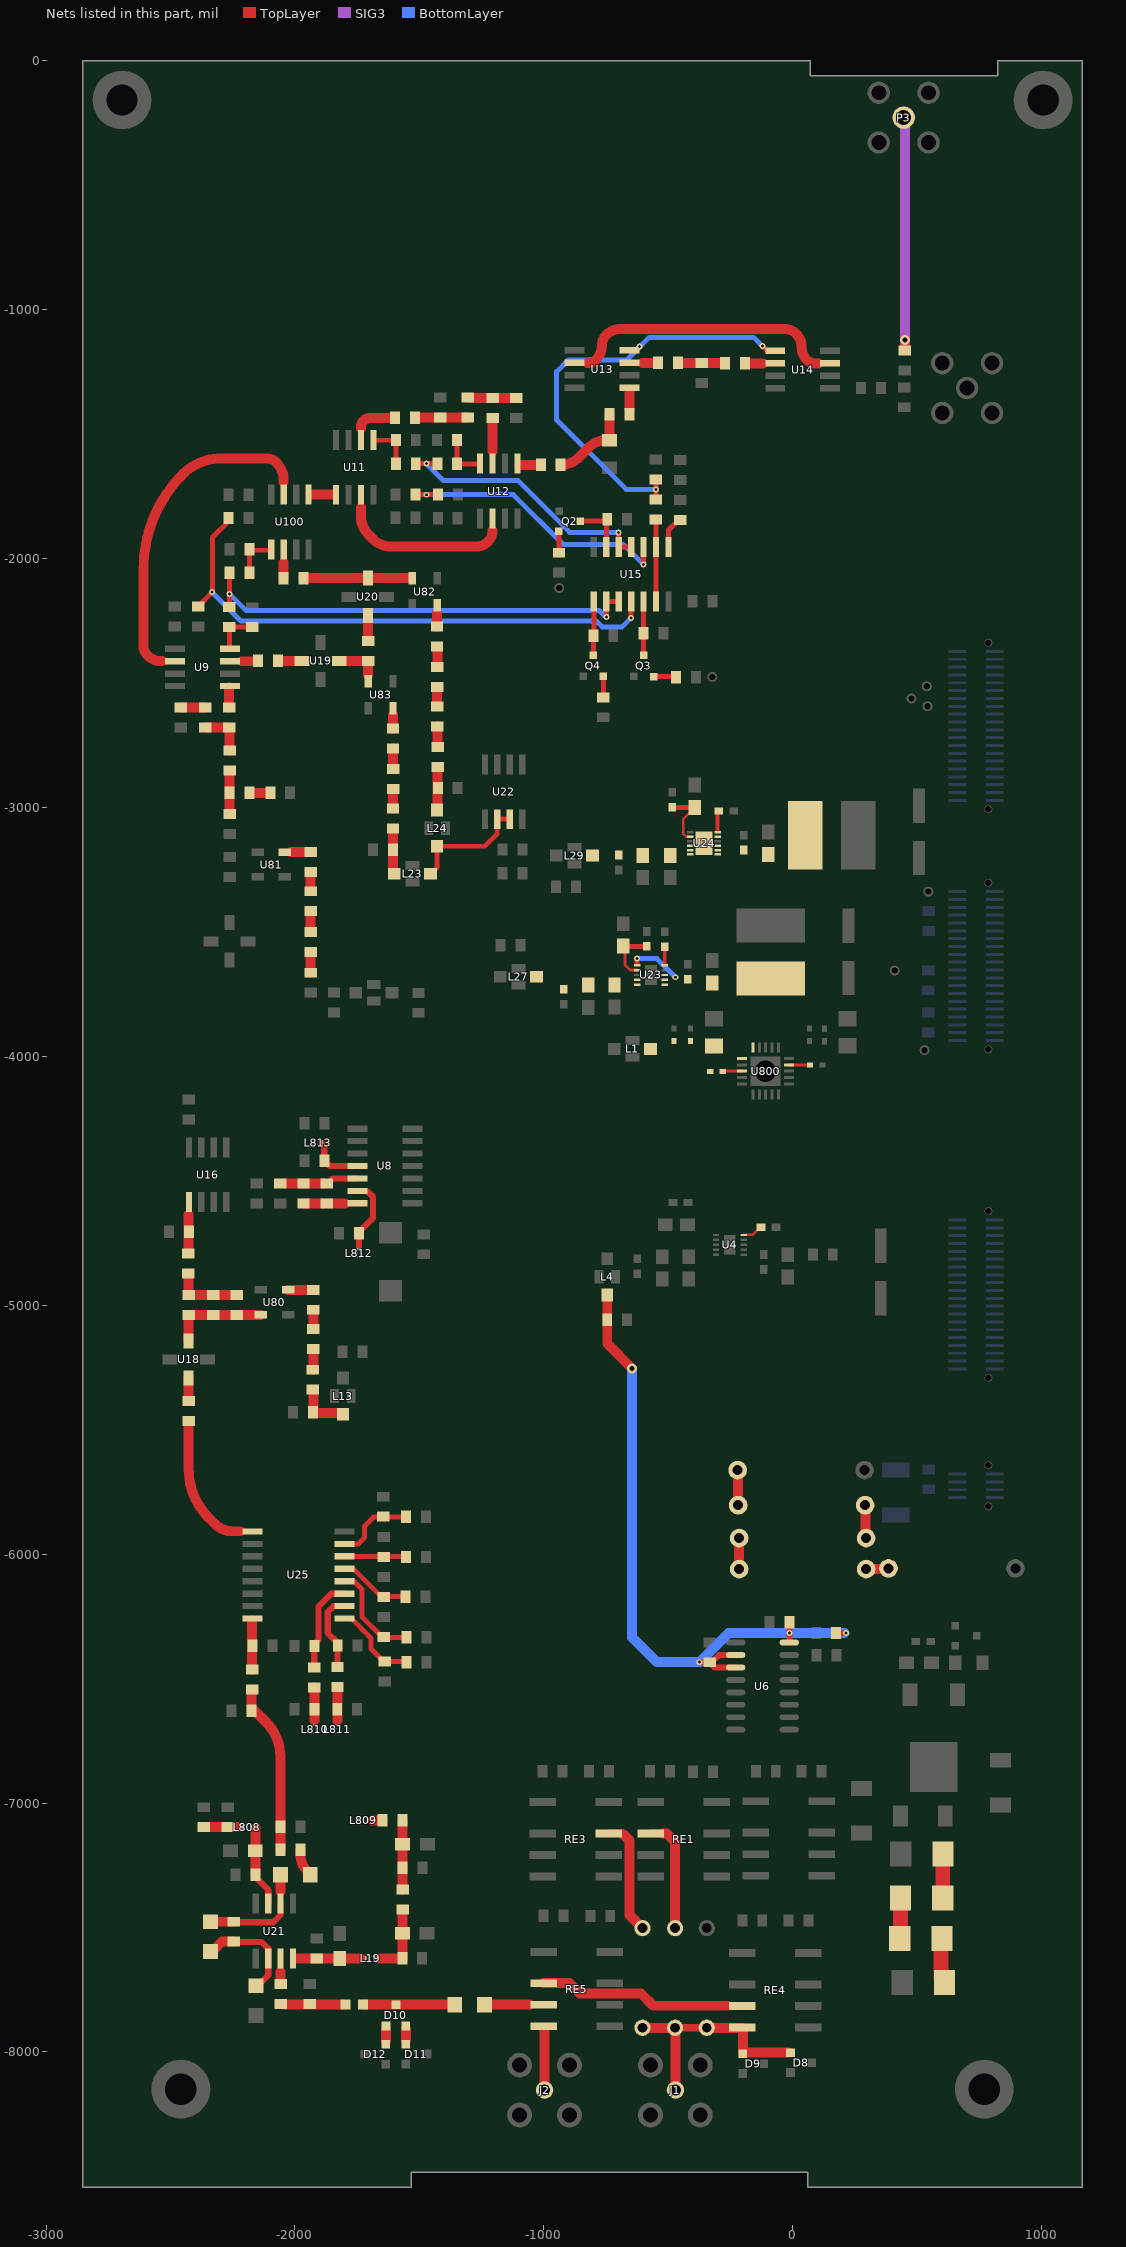
[diagram p0: the nets of this part, all layers, seen from the top]
# Altium PCB MISC109560.PcbDoc (part 6 of 7)
Units mil, origin at the board's own origin, x right, y up, seen from the top; angles counter-clockwise.
Board outline 4015.75 x 8543.31 mil, 4 copper layers (TopLayer, GND, SIG3, BottomLayer); 280 components, 173 nets, 936 pads, 3695 vias.

## Via types
v1: diameter 24, hole 12, TopLayer to BottomLayer, 3659 vias
v2: diameter 20, hole 12, TopLayer to BottomLayer, 32 vias
v3: diameter 40, hole 20, TopLayer to BottomLayer, 4 vias

## Nets (pads, with @x,y where several pads share a name; then routed paths per layer and width w, separated by ;. In a path a pad name is that pad's centre, name@x,y a point inside that pad or via, vN(x,y) a via of type N, cw(c..) or ccw(c..) an arc to the next point about the centre after c; other vN are vias at no path point) (continued)
NetC53_1: C53.1 C54.1 L15.1 | length 318.4
  TopLayer w40: C53.1@-932,-1623 -930.42,-1623 ccw(c-930.42,-1523) -859.71,-1593.71 -819.29,-1553.29 cw(c-748.58,-1624) -748.58,-1524 L15.1@-737,-1524 ; L15.1@-736,-1511 C54.1@-736,-1420
NetC53_2: C53.2 U12.1 | length 71
  TopLayer w40: U12.1@-1097,-1623 C53.2@-1026,-1623
NetC54_2: C54.2 U13.1 | length 72.6
  TopLayer w40: C54.2@-656,-1396.31 U13.1@-656,-1323.68
NetC55_1: C55.1 U13.3 | length 62.4
  TopLayer w40: -603.41,-1213.09 C55.1@-540.96,-1213.09
NetC55_2: C55.2 C56.1 L16.2 | length 182.1
  TopLayer w40: C55.2@-455.63,-1214.68 L16.2@-370,-1214.68 ; L16.2@-372,-1214.68 C56.1@-275.55,-1214.68
NetC56_2: C56.2 U14.6 | length 66.4
  TopLayer w40: C56.2@-185.96,-1216.09 -119.59,-1216.09
NetC57_1: C57.1 R41.1 U13.4 U14.5 | length 1839.7
  TopLayer w20: U13.4@-655.96,-1163.09 -629.41,-1163.09 -614,-1147.68 v1(-615,-1147.68) ; R41.1@-550,-1763.31 v1(-550,-1721.31) C57.1@-550,-1689.31 ; v1(-122,-1145.68) -102.59,-1165.09 U14.5@-69.96,-1165.09
  BottomLayer w20: -643,-1721.31 -603,-1721.31 ; v1@-608.5,-1142.18 -607,-1140.68 v1@-606,-1140.68 ; v1@-608,-1142.68 v1@-609,-1143.68 ; v1@-550,-1722.31 v1@-551,-1721.31 ; v1(-550,-1721.31) v1@-551,-1721.31 ; v1@-123,-1143.68 -126,-1140.68 v1@-127,-1140.68 ; v1(-122,-1145.68) v1@-127,-1140.68 ; v1@-609,-1143.68 -667,-1201.68 -901,-1201.68 -948,-1248.68 -948,-1442.68 -669.37,-1721.31 -603,-1721.31 ; v1@-609,-1143.68 v1@-606,-1140.68 ; v1@-606,-1140.68 -576,-1110.68 -157,-1110.68 v1@-127,-1140.68 ; -603,-1721.31 v1@-551,-1721.31
NetC58_1: C58.1 C65.1 | length 72
  TopLayer w40: C58.1@-2182,-2941.31 C65.1@-2110,-2941.31
NetC58_2: C58.2 L10.1 L11.1 | length 164.4
  TopLayer w40: L10.1@-2261.96,-3026.72 L11.1@-2261.96,-2862.31
NetC59_1: C59.1 L11.2 L12.1 | length 181.7
  TopLayer w40: C59.1@-2352,-2678.31 -2265,-2678.31 -2261.96,-2681.35 L11.2@-2261.96,-2771.72
NetC59_2: C59.2 C66.2 | length 98.6
  TopLayer w40: C66.2@-2459.59,-2597.72 C66.2@-2458.96,-2597.72 C59.2@-2360.96,-2597.72
NetC60_1: C60.1 R42.1 U9.4 | length 166.3
  TopLayer w20: U9.4@-2263.59,-2354.9 R42.1@-2263.59,-2274.27 C60.1@-2177.96,-2274.27
NetC61_2: C61.2 R43.2 U100.5 | length 173
  TopLayer w20: R43.2@-2183,-2056.31 -2183,-1966.31 U100.5@-2100,-1966.31
NetC62_2: C62.2 R44.1 U11.5 | length 171.3
  TopLayer w20: U11.5@-1672,-1524.31 -1595,-1524.31 -1594.41,-1524.9 R44.1@-1594.41,-1618.35
NetC63_2: C63.2 R45.1 U12.4 | length 181.1
  TopLayer w20: C63.2@-1348.41,-1523.35 -1348.41,-1614.72 -1342.82,-1620.31 U12.4@-1261,-1620.31
NetC64_2: C64.2 L13.3 R46.2 | length 191.2
  TopLayer w40: R46.2@-1927,-5347.26 -1926,-5348.26 C64.2@-1926,-5435 ; C64.2@-1926,-5433 L13.3@-1823,-5433
NetC67_1: C67.1 U18.1 | length 81.6
  TopLayer w40: C67.1@-2426.92,-5374.27 U18.1@-2426.92,-5292.72
NetC67_2: C67.2 U25.1 | length 555.4
  TopLayer w40: C67.2@-2426.96,-5465.31 -2426.96,-5658.26 ccw(c-2149.86,-5658.26) -2345.8,-5854.2 -2321.29,-5878.71 ccw(c-2250.58,-5808) -2250.58,-5908 -2219,-5908
NetC68_1: C68.1 C69.2 R49.2 R50.2 | length 269
  TopLayer w40: C69.2@-2426.96,-4881.31 C68.1@-2426.96,-4959.31 R49.2@-2235.96,-4959.31
NetC68_2: C68.2 R49.1 R50.1 U18.3 U80.1 | length 389.7
  TopLayer w40: U18.3@-2426.92,-5142.72 -2426.92,-5043.35 -2421.88,-5038.31 R50.1@-2328.96,-5038.31 R49.1@-2233.96,-5038.31 ; R49.1@-2232.26,-5038.31 U80.1@-2136.96,-5038.31
NetC69_1: C69.1 R53.2 U16.1 | length 152
  TopLayer w40: C69.1@-2426.96,-4787.31 -2426.96,-4635.31
NetC70_2: C70.2 C74.2 L18.1 L19.1 | length 273.5
  TopLayer w40: -1663,-7624 C74.2@-1574.48,-7624 ; C74.2@-1568.48,-7624 C70.2@-1568.48,-7523 L18.1@-1568.48,-7439
NetC71_2: C71.2 C75.2 L19.3 U21.4 | length 264
  TopLayer w40: U21.4@-1997.48,-7624 C75.2@-1912.48,-7624 C71.2@-1820.48,-7624 -1733.48,-7624
NetC72_1: C72.1 C73.2 L17.2 L18.2 | length 270
  TopLayer w40: L18.2@-1567.48,-7348 C72.1@-1567.48,-7260 C73.2@-1567.48,-7166 L17.2@-1567.48,-7078
NetC76_1: C76.1 U9.3 | length 54
  TopLayer w40: -2212,-2412.31 C76.1@-2158,-2412.31
NetC76_2: C76.2 U19.1 | length 84
  TopLayer w40: C76.2@-2065,-2411.31 U19.1@-1981,-2411.31
NetC77_1: C77.1 U19.3 U83.1 | length 165.7
  TopLayer w40: U19.3@-1822,-2411.31 C77.1@-1713,-2411.31 ; U83.1@-1706,-2468 C77.1@-1706,-2411.31
NetC77_2: C77.2 U20.1 | length 94
  TopLayer w40: C77.2@-1707,-2322.31 U20.1@-1707,-2228.31
NetC78_1: C78.1 U20.3 U82.1 | length 424.3
  TopLayer w40: C78.1@-1965,-2078.31 U20.3@-1707,-2078.31 U82.1@-1540.69,-2078.31
NetC78_2: C78.2 U100.6 | length 60.4
  TopLayer w40: C78.2@-2045,-2077.76 -2045,-2017.31
NetC79_1: C79.1 D10.3 R40.2 | length 369.5
  TopLayer w40: C79.1@-1727,-7810 R40.2@-1357.48,-7810
NetC79_2: C79.2 R58.2 R59.2 | length 237.1
  TopLayer w40: R58.2@-2044.07,-7809.41 C79.2@-1807,-7809.41
NetC80_2: C80.2 L20.2 L21.2 | length 204.4
  TopLayer w40: L20.2@-1513,-1433.31 L21.2@-1308.59,-1433.31
NetC81_2: C81.2 L21.1 L22.1 | length 184
  TopLayer w40: L21.1@-1295,-1354.31 C81.2@-1111,-1354.31
NetC82_1: C82.1 R60.2 | length 103.4
  TopLayer w40: C82.1@-1978.48,-7188 -1978.48,-7204.1 ccw(c-1878.48,-7204.1) -1949.19,-7274.81 R60.2@-1943,-7281
NetC82_2: C82.2 C116.1 R74.2 R82.2 | length 666.6
  TopLayer w40: R82.2@-2173.71,-6631 -2173.71,-6562.72 cw(c-2164.22,-6562.72) C116.1@-2170.93,-6556.01 ; R82.2@-2164,-6627 -2115.23,-6675.77 cw(c-2252.25,-6812.78) -2058.48,-6812.78 R74.2@-2058.48,-7095 ; C82.2@-2058.26,-7187.69 R74.2@-2058.26,-7100.22
NetC83_1: C83.1 C86.1 L808.1 U21.7 | length 407.3
  TopLayer w10: -2174,-7129 -2174,-7093 -2144,-7093 -2144,-7129
  TopLayer w25: C83.1@-2157.48,-7299 -2107.44,-7349.04 U21.7@-2107.44,-7404.41
  TopLayer w40: C86.1@-2159.26,-7191.41 -2159.26,-7108 ; C83.1@-2158.26,-7284.78 C86.1@-2158.26,-7189
NetC84_1: C84.1 L23.3 R62.2 | length 149.3
  TopLayer w40: L23.3@-1606,-3249 C84.1@-1606,-3174 ; C84.1@-1606,-3169.31 R62.2@-1606,-3095
NetC85_2: C85.2 L24.3 R65.1 | length 159.4
  TopLayer w40: L24.3@-1427,-3004.98 R65.1@-1427,-2845.61
NetC87_1: C87.1 R60.1 R69.1 U21.6 | length 418.7
  TopLayer w25: C87.1@-2263.48,-7479 -2122.48,-7479 -2087.48,-7479 -2057.48,-7449 -2057.48,-7426 U21.6@-2057.44,-7404.41
  TopLayer w40: R69.1@-2339.48,-7477 C87.1@-2251.48,-7477 ; -2058.09,-7355.39 R60.1@-2058.09,-7287.69
NetC87_2: C87.2 R61.2 R69.2 U21.2 | length 380
  TopLayer w25: C87.2@-2240.48,-7558 -2134.48,-7558 -2107.44,-7585.04 U21.2@-2107.44,-7624.41 -2107.44,-7691.96 R61.2@-2135.48,-7720
  TopLayer w40: R69.2@-2326,-7590 -2293,-7557 C87.2@-2250.48,-7557
NetC89_1: C89.1 L813.1 U8.11 | length 251.4
  TopLayer w10: L813.1@-1889.52,-4342 -1875,-4342 ; -1881.96,-4349 -1875,-4342.48 -1875,-4357
  TopLayer w25: C89.1@-1882,-4424.04 -1882,-4354 ; C89.1@-1882,-4419 C89.1@-1881.96,-4419.04 ; C89.1@-1881.96,-4419.31 C89.1@-1881.96,-4419.04 ; U8.11@-1748.37,-4440.35 -1860.65,-4440.35 C89.1@-1881.96,-4419.04
NetC90_1: C90.1 L32.2 L811.1 | length 134
  TopLayer w40: -1828.93,-6668 L32.2@-1828.93,-6534.01
NetC93_2: C93.2 C98.1 C99.2 L27.1 U23.9 U23.10
NetC94_2: C94.2 C95.1 L26.1 U23.1 U23.2 U23.3 U23.6 | length 205
  TopLayer w20: -625.14,-3627 v1(-625.14,-3607.14)
  BottomLayer w20: v1(-625.14,-3607.14) -545.86,-3607.14 v1(-471,-3682)
NetC96_1: C96.1 R70.1 U25.15 | length 298.6
  TopLayer w20: U25.15@-1792,-5959 -1746,-5959 -1720,-5933 -1720,-5887 -1683.69,-5850.69 R70.1@-1565.24,-5850.69
NetC101_1: C101.1 R72.1 U23.7 | length 203.2
  TopLayer w10: C101.1@-692,-3575 C101.1@-685,-3575
  TopLayer w12: C101.1@-674,-3580 -674,-3633 -653.75,-3653.25 U23.7@-625.14,-3653.25
  TopLayer w20: C101.1@-672,-3558 R72.1@-586,-3558
NetC102_1: C102.1 R73.1 U25.14 | length 244.4
  TopLayer w20: U25.14@-1800.71,-6008.69 R73.1@-1556.31,-6008.69
NetC104_1: C104.1 L812.1 U8.13 | length 294.8
  TopLayer w25: U8.13@-1748.37,-4540.35 -1710.65,-4540.35 -1686,-4565 -1686,-4648 -1742,-4704 -1742,-4764
NetC105_2: C105.2 L31.1 L810.1 | length 133
  TopLayer w40: -1921.93,-6669 L31.1@-1921.93,-6536.01
NetC109_1: C109.1 R75.1 U25.13 | length 276.1
  TopLayer w20: U25.13@-1800.71,-6058.69 U25.13@-1796,-6058.69 ; U25.13@-1796,-6057 -1767,-6057 -1695,-6129 C109.1@-1655,-6169 ; C109.1@-1657.93,-6171.01 R75.1@-1573.93,-6171.01
NetC110_2: C110.2 C113.1 C114.2 L29.1 U24.10 U24.11 U24.12
NetC111_2: C111.2 C112.1 L28.1 U24.1 U24.2 U24.3 U24.5 U24.13
NetC116_2: C116.2 R83.2 U25.8 | length 197.3
  TopLayer w40: U25.8@-2171.93,-6271.01 cw(c-2172.46,-6271.54) -2171.71,-6271.54 ; C116.2@-2171.71,-6463.69 U25.8@-2171.71,-6267.01
NetC118_1: C118.1 R77.1 U25.12 | length 399.3
  TopLayer w20: U25.12@-1800.71,-6108.69 U25.12@-1792,-6108.69 ; U25.12@-1792,-6108 -1763,-6108 -1731,-6140 -1731,-6251 -1648,-6334 R77.1@-1560,-6334
NetC119_1: C119.1 R81.1 U24.8 | length 243.4
  TopLayer w10: -435.5,-3109.53 -429.06,-3115.98 ; -435.5,-3109.5 -440,-3105 -440,-3047 C119.1@-393,-3000 ; -429.02,-3115.98 -427.26,-3117.74 U24.8@-411.41,-3117.74
  TopLayer w20: R81.1@-478,-3000 C119.1@-393,-3000
NetC128_2: C128.2 L31.2 U25.11 | length 370.5
  TopLayer w25: L31.2@-1921.93,-6448.01 C128.2@-1921.93,-6369.01 -1921.93,-6361.01 -1904.93,-6344.01 -1904.93,-6210.01 -1853.61,-6158.69 U25.11@-1800.71,-6158.69
NetC129_2: C129.2 L32.1 U25.10 | length 385.6
  TopLayer w20: -1865.93,-6276.01 -1865.93,-6231.01 -1843.61,-6208.69 U25.10@-1800.71,-6208.69 ; L32.1@-1828.93,-6448.01 L32.1@-1828.93,-6439.01
  TopLayer w25: -1843.61,-6208.69 -1844.61,-6208.69 -1867.93,-6232.01 -1867.93,-6317.01 -1828.93,-6356.01 L32.1@-1828.93,-6439.01
NetC130_1: C130.1 R84.1 U25.9 | length 337.5
  TopLayer w20: U25.9@-1800.71,-6258.69 U25.9@-1772,-6258.69 ; U25.9@-1772,-6260 -1732,-6300 -1724,-6308 -1695,-6337 -1695,-6379 C130.1@-1647,-6427 ; C130.1@-1649.93,-6432.01 R84.1@-1559.93,-6432.01
NetC803_1: C803.1 U800.14 | length 77.1
  TopLayer w12: U800.14@-14.02,-4033.9 C803.1@63.1,-4033.9
NetC804_1: C804.1 C805.1 C806.1 L1.1 R800.1 U800.1 U800.20
NetC809_1: C809.1 L25.2 L808.3 | length 137
  TopLayer w40: L25.2@-2366,-7097 C809.1@-2269,-7097 -2229,-7097
NetD2_1: D2.1 D3.2 | length 145
  TopLayer w60: D2.1@596,-7702 D3.2@596,-7557
NetD3_1: D3.1 D4.2 | length 146.5
  TopLayer w60: D3.1@433,-7527.54 D4.2@433,-7381
NetD4_1: D4.1 D5.2 | length 146
  TopLayer w60: D4.1@603,-7381 D5.2@603,-7235
NetD8_1: D8.1 D9.1 J1.5 R17.1 R20.1 R23.1 RE4.4 | length 938.4
  TopLayer w30: R23.1@-603.26,-7903 R23.1@-594.59,-7903 ; R17.1@-472.26,-7903 R20.1@-345.26,-7903 ; RE4.4@-201,-7908.59 RE4.4@-201,-7903.87
  TopLayer w40: R23.1@-595,-7902.59 -594.59,-7903 -594.38,-7903.21 R17.1@-472.26,-7903.21 ; R17.1@-472.26,-7903 R17.1@-472.26,-7903.21 ; J1.5@-471.26,-8153.31 -471.26,-7904.21 R17.1@-472.26,-7903.21 ; R20.1@-345.26,-7903.21 RE4.4@-201.66,-7903.21 ; RE4.4@-198,-7908.59 -199.5,-7910.09 -199.5,-8003.09 D8.1@-13.96,-8003.09
NetD10_1: D10.1 D12.2 | length 49.8
  TopLayer w40: D12.2@-1634.26,-7956.78 D10.1@-1634.26,-7907
NetD10_2: D10.2 D11.1 | length 47.8
  TopLayer w40: D11.1@-1554.26,-7952.78 D10.2@-1554.26,-7905
NetJ2_5: J2.5 RE5.4 | length 247.3
  TopLayer w40: J2.5@-997,-8153.31 RE5.4@-997,-7906
NetL12_2: L12.2 U9.1 | length 79.4
  TopLayer w40: L12.2@-2263.96,-2597.72 U9.1@-2263.96,-2518.35
NetL17_1: L17.1 L809.3 | length 42.5
  TopLayer w40: -1690,-7070 L17.1@-1647.48,-7070
NetL20_1: L20.1 U11.6 | length 163.5
  TopLayer w40: -1735,-1477.31 -1735,-1471.86 cw(c-1697.44,-1471.86) -1724,-1445.31 cw(c-1697.54,-1471.77) -1697.54,-1434.35 L20.1@-1598.41,-1434.35
NetL22_2: L22.2 U12.3 | length 133.6
  TopLayer w40: -1205.41,-1567.9 L22.2@-1205.41,-1434.35
NetL23_1: L23.1 L24.1 U22.6 U22.7 | length 472.8
  TopLayer w20: L23.1@-1440,-3253 -1429,-3242 L24.1@-1429,-3155.61 -1236.61,-3155.61 -1187,-3106 U22.6@-1187,-3042 ; U22.6@-1181,-3047 U22.7@-1136.69,-3047
NetP3_5: P3.5 R1.2 | length 922
  TopLayer w40: R1.2@452,-1154 v3(452,-1122)
  SIG3 w40: v3@452,-1121 P3.5@452,-231
NetQ2_2: Q2.2 R51.1 | length 80
  TopLayer w20: R51.1@-939,-1976.31 Q2.2@-939,-1896.31
NetQ2_3: Q2.3 R54.2 U15.13 | length 199.4
  TopLayer w20: Q2.3@-846,-1849.31 R54.2@-750,-1849.31 ; U15.13@-748.96,-1952.72 R54.2@-748.96,-1849.35
NetQ3_2: Q3.2 R52.1 | length 81
  TopLayer w20: Q3.2@-558,-2474.31 R52.1@-477,-2474.31
NetQ3_3: Q3.3 R55.1 U15.5 | length 207.6
  TopLayer w20: Q3.3@-598.96,-2380.31 U15.5@-598.96,-2172.72
NetQ4_2: Q4.2 R56.2 | length 80
  TopLayer w20: R56.2@-761,-2557.31 Q4.2@-761,-2477.31
NetQ4_3: Q4.3 R57.2 U15.1 | length 187.6
  TopLayer w20: Q4.3@-801,-2378.31 R57.2@-801,-2309.31 ; R57.2@-798.96,-2291.27 -798.96,-2173.31 U15.1@-798.96,-2172.72
NetR7_1: R7.1 R8.1 | length 132
  TopLayer w40: R8.1@-219,-5803.31 R7.1@-219,-5671.31
NetR8_2: R8.2 R9.2 | length 112
  TopLayer w40: R9.2@292,-5928.31 R8.2@292,-5816.31
NetR9_1: R9.1 R10.1 | length 105.4
  TopLayer w40: R10.1@-214.78,-6059.94 R9.1@-214.78,-5954.53
NetR10_2: R10.2 R11.2 | length 78
  TopLayer w40: R10.2@295,-6058.94 326,-6058.94 369.63,-6058.94 R11.2@372,-6061.31
NetR13_1: R13.1 U4.5 | length 68.8
  TopLayer w10: U4.5@-197,-4717.57 -161.57,-4717.57 R13.1@-138,-4694
NetR17_2: R17.2 RE1.2 | length 458
  TopLayer w30: RE1.2@-569.66,-7121.98 RE1.2@-522,-7121.98
  TopLayer w40: RE1.2@-522,-7122.59 -506,-7122.59 -472.26,-7156.33 R17.2@-472.26,-7503
NetR23_2: R23.2 RE3.7 | length 471.1
  TopLayer w30: RE3.7@-739.31,-7121.98 -680.61,-7121.98
  TopLayer w40: -683,-7123.59 -655,-7151.59 -655,-7451.26 R23.2@-603.26,-7503
NetR27_2: R27.2 R28.1 U15.4 | length 2218.9
  TopLayer w20: R27.2@-2388.59,-2192.27 v1@-2332,-2135.68 ; v1(-2333,-2134.68) v1@-2332,-2135.68 ; R28.1@-2264,-1847.31 -2332,-1915.31 v1@-2332,-2135.68 ; v1(-648.96,-2238.35) U15.4@-648.96,-2172.72
  BottomLayer w20: v1(-2333,-2134.68) -2217.37,-2250.31 -789.69,-2250.31 -765.69,-2274.31 -685,-2274.31 v1@-650,-2239.31
NetR29_2: R29.2 R30.2 U15.10 | length 1144.6
  TopLayer w20: R29.2@-1508.96,-1742.35 v1@-1472,-1742.35 ; v1(-1472,-1743.31) v1@-1472,-1742.35 ; R30.2@-1425.41,-1742.35 v1@-1472,-1742.35 ; v1(-598.96,-2024.27) U15.10@-598.96,-1952.72
  BottomLayer w20: v1@-1471,-1743 -1122.31,-1743 -923,-1942.31 -680.92,-1942.31 v1(-598.96,-2024.27)
NetR31_2: R31.2 U15.8 | length 121.1
  TopLayer w20: U15.8@-498.96,-1952.72 -498.96,-1885.27 R31.2@-461,-1847.31
NetR33_1: R33.1 R34.1 U8.14 | length 139.4
  TopLayer w40: R33.1@-1965.41,-4590.31 R34.1@-1887.96,-4590.31 ; R34.1@-1860.92,-4590.35 -1798.96,-4590.35
NetR33_2: R33.2 R34.2 R35.2 U8.12 | length 278
  TopLayer w25: R34.2@-1864.96,-4508.31 -1847,-4490.35 U8.12@-1748.37,-4490.35
  TopLayer w40: R35.2@-2038.96,-4510.31 R34.2@-1884.96,-4510.31
NetR36_2: R36.2 R37.1 | length 74.4
  TopLayer w40: R36.2@-1937.27,-3664 R37.1@-1937.27,-3589.63
NetR37_2: R37.2 R38.2 | length 59
  TopLayer w40: R37.2@-1937.27,-3493 R38.2@-1937.27,-3434.04
NetR38_1: R38.1 R39.1 | length 66.1
  TopLayer w40: R38.1@-1937.27,-3336.41 R39.1@-1937.27,-3270.27
NetR39_2: R39.2 U81.3 | length 78
  TopLayer w40: -2015,-3179 R39.2@-1937,-3179
NetR40_1: R40.1 RE5.3 | length 182
  TopLayer w40: R40.1@-1238,-7810 -1056,-7810
NetR41_2: R41.2 U15.6 U15.9 | length 317.4
  TopLayer w20: U15.6@-548.96,-2172.72 U15.9@-548.96,-1952.72 R41.2@-548.96,-1855.35
NetR42_2: R42.2 R43.1 U15.2 U15.3 | length 1787.9
  TopLayer w20: R42.2@-2263.59,-2194.27 v1(-2263.59,-2141.72) R43.1@-2263.59,-2068.72 ; v1(-748.96,-2235.35) U15.2@-748.96,-2172.72 ; U15.2@-747.41,-2172.72 U15.3@-698.96,-2172.72
  BottomLayer w20: v1(-2263.59,-2141.72) -2196,-2209.31 -776.69,-2209.31 v1@-751,-2235
NetR44_2: R44.2 R45.2 U15.11 U15.12 | length 1059.7
  TopLayer w20: R44.2@-1505,-1618.31 v1(-1471,-1618.31) R45.2@-1428,-1618.31 ; U15.12@-698.96,-1952.72 v1(-698.96,-1894.27) ; U15.12@-691.59,-1952.72 U15.11@-648.96,-1952.72
  BottomLayer w20: v1@-1470,-1620 -1403,-1687 -1103.31,-1687 -896,-1894.31 v1@-702,-1894.31
NetR46_1: R46.1 R47.2 | length 80
  TopLayer w40: R46.1@-1925.48,-5258.53 R47.2@-1925.48,-5178.53
NetR47_1: R47.1 R48.1 | length 78
  TopLayer w40: R47.1@-1926,-5096 R48.1@-1926,-5018
NetR48_2: R48.2 U80.3 | length 95.5
  TopLayer w40: R48.2@-1933.31,-4938.31 U80.3@-2027.12,-4938.31 ; U80.3@-2027.12,-4938.31 cw(c-2026.38,-4939.05) -2026.38,-4938 ccw(c-2026.38,-4939.05) U80.3@-2027.12,-4938.31
NetR58_1: R58.1 U21.3 | length 48.4
  TopLayer w40: R58.1@-2057.44,-7727.41 -2057.44,-7678.96
NetR62_1: R62.1 R63.1 | length 71
  TopLayer w40: R62.1@-1605,-2996.31 R63.1@-1605,-2925.31
NetR63_2: R63.2 R64.2 | length 77
  TopLayer w40: R63.2@-1606,-2839.31 R64.2@-1606,-2762.31
NetR64_1: R64.1 U83.3 | length 53.3
  TopLayer w40: R64.1@-1606,-2682.31 -1606,-2629
NetR65_2: R65.2 R66.2 | length 83
  TopLayer w40: R65.2@-1427,-2757.61 R66.2@-1427,-2674.61
NetR66_1: R66.1 R67.1 | length 58
  TopLayer w40: R66.1@-1429,-2585.61 R67.1@-1429,-2527.61
NetR67_2: R67.2 R68.1 | length 67.6
  TopLayer w40: R67.2@-1428,-2435.61 R68.1@-1428,-2368
NetR68_2: R68.2 U82.3 | length 55.3
  TopLayer w40: R68.2@-1429,-2272.31 -1429,-2217
NetR71_1: R71.1 U23.5 | length 66
  TopLayer w16: U23.5@-514,-3630 R71.1@-514,-3564
NetR80_1: R80.1 U24.6 | length 81.7
  TopLayer w16: -302,-3095 R80.1@-302,-3013.31
NetR800_2: R800.2 U800.3 | length 70.5
  TopLayer w12: R800.2@-273.51,-4059.49 U800.3@-203,-4059.49
NetRE4_3: RE4.3 RE5.2 | length 836.5
  TopLayer w30: -262,-7816.6 RE4.3@-201.66,-7816.6
  TopLayer w40: RE5.2@-1000.66,-7723.98 -897.39,-7723.98 -855.64,-7765.73 -608.86,-7765.73 -560,-7814.59 -262,-7814.59
NetU9_6: U9.6 U100.3 | length 1323.8
  TopLayer w40: -2533.01,-2412.1 cw(c-2537.98,-2337.29) -2591,-2390.31 cw(c-2549.96,-2349.27) -2608,-2349.27 -2608,-2040.27 cw(c-2072.13,-2040.27) -2451.05,-1661.35 cw(c-2296.42,-1815.98) -2296.42,-1597.31 -2113.63,-1597.31 cw(c-2113.63,-1651.93) -2075,-1613.31 cw(c-2147.43,-1685.73) -2045.21,-1692.29
NetU11_1: U11.1 U100.1 | length 87.6
  TopLayer w40: U100.1@-1933,-1742.72 U11.1@-1845.41,-1742.72
NetU11_3: U11.3 U12.6 | length 667.1
  TopLayer w40: -1734.41,-1794.31 -1734.41,-1831.48 ccw(c-1634.41,-1831.48) -1705.12,-1902.19 -1685.29,-1922.02 ccw(c-1614.58,-1851.31) -1614.58,-1951.31 -1270.87,-1951.31 ccw(c-1270.87,-1886.44) -1225,-1932.31 -1224.38,-1931.69 ccw(c-1268.77,-1887.31) -1206,-1887.31
NetU13_6: U13.6 U14.3 | length 1090.9
  TopLayer w40: -824,-1213.09 -818.55,-1213.09 ccw(c-818.55,-1174.13) -791,-1201.68 ccw(c-848.94,-1143.74) -767,-1143.74 cw(c-706.5,-1143.74) -749.28,-1100.96 cw(c-690.66,-1159.58) -690.66,-1076.68 -32.87,-1076.68 cw(c-32.87,-1141.55) 13,-1095.68 15.49,-1098.17 cw(c-34.01,-1147.68) 36,-1147.68 36,-1152.39 ccw(c104.28,-1152.39) 56,-1200.68 ccw(c92.21,-1164.46) 92.21,-1215.68 ccw(c94.63,-1213.26) 94.63,-1216.68 104,-1216.68
VCC: C13.1 C15.2 L4.3 R15.1 R16.2 U6.2 U6.3 U6.16 | length 2709.5
  TopLayer w24: v1(-375.31,-6434.31) R15.1@-334,-6434.31 ; R15.1@-327,-6442 -313.69,-6455.31 U6.3@-229,-6455.31 ; R15.1@-312,-6422 -295.31,-6405.31 U6.2@-229,-6405.31 ; U6.16@-13,-6349 C15.2@-13,-6275.1 ; R16.2@174.8,-6316.81 v1(215.19,-6316.81)
  TopLayer w30: C15.2@-13,-6273.69 -13,-6275.1 C15.2@-12.8,-6274.9
  TopLayer w40: L4.3@-745,-4958.67 C13.1@-745,-5059 -745,-5154 v3(-645,-5254)
  BottomLayer w40: v3(-645,-5254) -645,-6334 -545,-6434 v1@-372,-6434 ; v1@-372,-6432 -257,-6317 v1(-12,-6317) v1@208,-6317
pads on no net: D1.1 D8.3 D9.3 D11.3 D12.3 P1.0 P1.1 P1.2 P1.3 P1.4 P1.7 P1.8 P1.9 P1.10 P1.13 P1.14 P1.15 P1.16 P1.19 P1.21 P1.22 P1.25 P1.27 P1.31 P2.0 P4.0 P4.1 P4.3 P4.7 P4.9 P4.13 P4.15 P4.19 P4.20 P4.21 P4.25 P4.27 P4.31 P4.33 P4.37 P4.38 P4.39 P4.40 P5.0 RE1.4 RE1.5 RE1.6 RE1.7 RE2.2 RE2.3 RE2.4 RE2.5 RE3.2 RE3.3 RE3.4 RE3.5 RE4.5 RE4.6 RE4.7 RE5.5 RE5.6 RE5.7 U4.4 U6.4 U6.5 U6.7 U6.9 U6.11 U6.12 U8.6 U21.1 U21.5 U21.8 U22.3 U23.4 U24.4 U24.7 U80.2 U80.4 U81.2 U81.4 U82.2 U82.4 U83.2 U83.4 U800.2 U800.4 U800.8 U800.10 U800.12 U800.17 U800.18 U800.19
copper on no net:
  other v1: 768,-8198.31 683,-8197.31

## Polygon pours and split planes (outlines as drawn)
GND on TopLayer "Bottom Layer-No Net" (solid, remove dead copper, pour order 1020): -3191,-3960 -3191,-8552 -3011,-8732 -2847,-8896 -2458,-8896 1357,-8896 1387,-8866 1806,-8447 1806,-8223 1806,-6391 1787,-6372 1649,-6234 789,-6234 -267,-6234 -339,-6162 -362,-6139 -362,-6071 -362,-5565 -265,-5468 -255,-5458 -219,-5458 1268,-5458 1308,-5418 1387,-5339 1387,-5250 1387,214 1372,229 1013,588 -244,588 -2473,588 -2682,379 -3191,-130 -3191,-3960
NetC6_1 on TopLayer "Bottom Layer-No Net" (solid, remove dead copper, pour order 1000): 229,-6889 229,-6912 229,-6966 233,-6970 236,-6973 243,-6973 558,-6973 569,-6984 578,-6993 578,-7029 578,-7092 581,-7095 586,-7100 593,-7100 674,-7100 677,-7097 687,-7087 687,-7014 687,-6905 697,-6895 729,-6863 835,-6863 879,-6863 882,-6863 894,-6851 910,-6835 910,-6812 910,-6783 905,-6778 882,-6755 614,-6755 266,-6755 236,-6785 229,-6792 229,-6889
NetC7_2 on TopLayer "Bottom Layer-No Net" (solid, remove dead copper, pour order 1001): -782,-4765 -782,-4810 -778,-4814 -757,-4835 -521,-4835 -301,-4835 -299,-4833 -295,-4829 -295,-4792 -295,-4773 -296,-4772 -297,-4771 -302,-4771 -374,-4771 -390,-4755 -397,-4748 -476,-4748 -772,-4748 -781,-4757 -782,-4758 -782,-4764
A6V on TopLayer "Bottom Layer-No Net" (solid, remove dead copper, pour order 1002): 138,-4760 138,-4817 144,-4823 153,-4832 296,-4832 389,-4832 401,-4820 414,-4807 414,-4791 414,-4600 407,-4593 400,-4586 377,-4586 179,-4586 163,-4602 138,-4627 138,-4760
NetC8_2 on TopLayer "Bottom Layer-No Net" (solid, remove dead copper, pour order 1003): -325,-4699 -325,-4719 -323,-4721 -321,-4723 -316,-4723 -297,-4723 -296,-4722 -295,-4721 -295,-4719 -295,-4667 -288,-4660 -260,-4632 -203,-4632 -26,-4632 -18,-4640 -11,-4647 -11,-4666 -11,-4725 -14,-4728 -38,-4752 -185,-4752 -208,-4752 -209,-4753 -210,-4754 -210,-4758 -210,-4799 -209,-4800 -195,-4814 -112,-4814 -75,-4814 -64,-4825 -61,-4828 -6,-4828 93,-4828 98,-4823 101,-4820 101,-4813 101,-4740 98,-4737 95,-4734 78,-4734 30,-4734 24,-4728 13,-4717 13,-4688 13,-4629 1,-4617 -5,-4611 -43,-4611 -272,-4611 -314,-4653 -325,-4664 -325,-4699
+12.5V on TopLayer "Bottom Layer-No Net" (solid, remove dead copper, pour order 1004): -65,-3945 -65,-3957 -65,-3983 -63,-3985 -62,-3986 -58,-3986 -44,-3986 -40,-3990 -35,-3995 -35,-4003 -35,-4012 -33,-4014 -32,-4015 -29,-4015 167,-4015 170,-4018 170,-4022 170,-4050 168,-4052 167,-4053 8,-4053 -33,-4053 -34,-4054 -34,-4055 -34,-4064 -33,-4065 -32,-4066 -29,-4066 569,-4066 573,-4062 590,-4045 590,-3953 563,-3926 96,-3926 -57,-3926 -62,-3931 -65,-3934 -65,-3945
NetC804_1 on TopLayer "Bottom Layer-No Net" (solid, remove dead copper, pour order 1005): -597,-3943 -597,-4006 -591,-4012 -579,-4024 -497,-4024 -370,-4024 -363,-4031 -358,-4036 -358,-4052 -358,-4068 -353,-4073 -352,-4074 -342,-4074 -320,-4074 -318,-4072 -317,-4071 -317,-4065 -317,-4038 -307,-4028 -294,-4015 -212,-4015 -184,-4015 -183,-4014 -183,-4011 -183,-3991 -180,-3988 -178,-3986 -163,-3986 -154,-3986 -153,-3985 -153,-3979 -153,-3932 -157,-3928 -159,-3926 -317,-3926 -590,-3926 -596,-3932 -597,-3933 -597,-3942
A6V on TopLayer "Bottom Layer-No Net" (solid, remove dead copper, pour order 1006): -236,-3389 -236,-3533 -226,-3543 -221,-3548 -185,-3548 302,-3548 326,-3572 337,-3583 337,-3622 337,-3663 345,-3671 354,-3680 383,-3680 452,-3680 458,-3674 475,-3657 475,-3620 475,-3462 374,-3361 368,-3355 36,-3355 -202,-3355 -236,-3389
NetC94_2 on TopLayer "Bottom Layer-No Net" (solid, remove dead copper, pour order 1007): -528,-3675 -528,-3690 -528,-3751 -523,-3756 -488,-3791 -285,-3791 40,-3791 54,-3777 60,-3771 60,-3760 60,-3625 58,-3623 50,-3615 -192,-3615 -221,-3615 -250,-3644 -278,-3672 -431,-3672 -455,-3672 -458,-3669 -459,-3668 -504,-3668 -526,-3668 -527,-3669 -528,-3670 -528,-3675
NetC93_2 on TopLayer "Bottom Layer-No Net" (solid, remove dead copper, pour order 1008): -1058,-3694 -1058,-3735 -1055,-3738 -1045,-3748 -884,-3748 -625,-3748 -619,-3742 -612,-3735 -612,-3717 -612,-3689 -613,-3688 -614,-3687 -622,-3687 -660,-3687 -674,-3673 -697,-3650 -870,-3650 -1050,-3650 -1054,-3654 -1058,-3658 -1058,-3694
-5.4V on TopLayer "Bottom Layer-No Net" (solid, remove dead copper, pour order 1009): 191,-2997 191,-3270 212,-3291 223,-3302 292,-3302 374,-3302 438,-3366 454,-3382 535,-3382 569,-3382 576,-3375 588,-3363 588,-3349 588,-3167 566,-3145 553,-3132 522,-3132 443,-3132 430,-3119 412,-3101 412,-3046 412,-2995 396,-2979 383,-2966 349,-2966 200,-2966 195,-2971 191,-2975 191,-2997
NetC111_2 on TopLayer "Bottom Layer-No Net" (solid, remove dead copper, pour order 1010): -390,-3102 -390,-3244 -382,-3252 -317,-3317 -14,-3317 103,-3317 117,-3303 130,-3290 130,-3246 130,-2973 123,-2966 115,-2958 89,-2958 -7,-2958 -16,-2967 -33,-2984 -33,-3039 -33,-3143 -41,-3151 -43,-3153 -199,-3153 -222,-3153 -226,-3149 -227,-3148 -288,-3148 -317,-3148 -319,-3146 -322,-3143 -322,-3139 -322,-3128 -319,-3125 -318,-3124 -313,-3124 -287,-3124 -286,-3123 -286,-3120 -286,-3114 -287,-3113 -288,-3112 -291,-3112 -318,-3112 -321,-3109 -322,-3108 -322,-3101 -322,-3094 -323,-3093 -325,-3091 -329,-3091 -385,-3091 -388,-3094 -390,-3096 -390,-3101